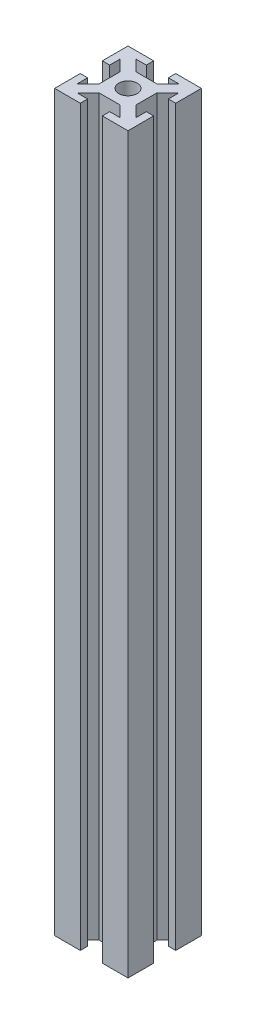
SolidWorks part; units mm, degrees
ref_plane "Front Plane" through (0, 0, 0) normal (0, 0, 1) x (1, 0, 0)
ref_plane "Top Plane" through (0, 0, 0) normal (0, 1, 0) x (1, 0, 0)
ref_plane "Right Plane" through (0, 0, 0) normal (1, 0, 0) x (0, 0, -1)
other "Configuration Table"
sketch "Sketch1" plane through (0, 0, 0) normal (0, 1, 0) x (1, 0, 0)
  line L0 (-6, 20) -> (-6, 16)
  line L5 (-20, 20) -> (-6, 20)
  line L6 (-20, 20) -> (-20, 6)
  line L7 (-20, -20) -> (-6, -20)
  line L8 (20, 20) -> (20, 6)
  line L9 (-20, 20) -> (20, -20) construction
  line L10 (-20, -20) -> (20, 20) construction
  line L11 (-6, 16) -> (-11.7574, 16)
  line L12 (-11.7574, 16) -> (-5.7574, 10)
  line L13 (5.7574, 10) -> (11.7574, 16)
  line L14 (11.7574, 16) -> (6, 16)
  line L15 (6, 16) -> (6, 20)
  line L16 (20, 6) -> (16, 6)
  line L17 (16, 6) -> (16, 11.7574)
  line L18 (16, 11.7574) -> (10, 5.7574)
  line L19 (10, -5.7574) -> (16, -11.7574)
  line L20 (16, -11.7574) -> (16, -6)
  line L21 (16, -6) -> (20, -6)
  line L22 (6, -20) -> (6, -16)
  line L23 (6, -16) -> (11.7574, -16)
  line L24 (11.7574, -16) -> (5.7574, -10)
  line L25 (-5.7574, -10) -> (-11.7574, -16)
  line L26 (-11.7574, -16) -> (-6, -16)
  line L27 (-6, -16) -> (-6, -20)
  line L28 (-20, -6) -> (-16, -6)
  line L29 (-16, -6) -> (-16, -11.7574)
  line L30 (-16, -11.7574) -> (-10, -5.7574)
  line L31 (-10, 5.7574) -> (-16, 11.7574)
  line L32 (-16, 11.7574) -> (-16, 6)
  line L33 (-16, 6) -> (-20, 6)
  line L34 (6, 20) -> (20, 20)
  line L35 (-20, -6) -> (-20, -20)
  line L36 (20, -6) -> (20, -20)
  line L37 (6, -20) -> (20, -20)
  line L39 (-5.7574, -10) -> (5.7574, -10)
  line L40 (-10, -5.7574) -> (-10, 5.7574)
  line L41 (-5.7574, 10) -> (5.7574, 10)
  line L42 (10, -5.7574) -> (10, 5.7574)
  line L43 (-10, -10) -> (10, 10) construction
  line L44 (-10, 10) -> (10, -10) construction
  circle A0 centre (0, 0) radius 5
  point P0 (0, 0)
  point P5 (0, 0)
  point P37 (0, 0)
  dimension "D10" = 10
  dimension "D1" = 40
  dimension "D2" = 4
  dimension "D3" = 4
  dimension "D4" = 14
  dimension "D5" = 14
  dimension "D6" = 3
  dimension "D7" = 3
  dimension "D8" = 4
  dimension "D9" = 20
extrude "Boss-Extrude1" add sketch "Sketch1" along normal blind 400
